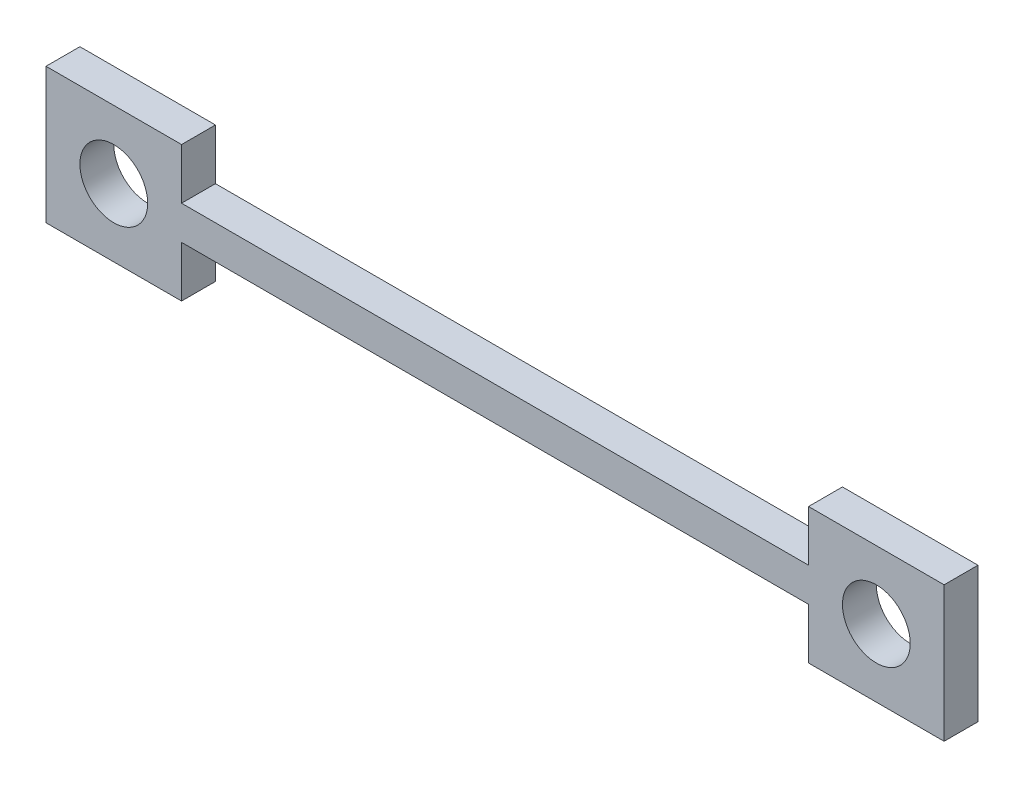
SolidWorks part; units mm, degrees
ref_plane "Front Plane" through (0, 0, 0) normal (0, 0, 1) x (1, 0, 0)
ref_plane "Top Plane" through (0, 0, 0) normal (0, 1, 0) x (1, 0, 0)
ref_plane "Right Plane" through (0, 0, 0) normal (1, 0, 0) x (0, 0, -1)
sketch "Sketch1" plane through (0, 0, 0) normal (0, 0, 1) x (1, 0, 0)
  line L0 (200, 50) -> (2050, 50)
  line L1 (-200, 200) -> (200, 200)
  line L2 (-200, 200) -> (-200, -200)
  line L3 (-200, -200) -> (200, -200)
  line L4 (200, 200) -> (200, 50)
  line L5 (200, -50) -> (2050, -50)
  line L6 (200, -50) -> (200, -200)
  line L7 (2050, -50) -> (2050, -200)
  line L9 (2050, 200) -> (2450, 200)
  line L10 (2050, 200) -> (2050, 50)
  line L11 (2050, -200) -> (2450, -200)
  line L12 (2450, 200) -> (2450, -200)
  circle A0 centre (0, 0) radius 100
  circle A1 centre (2250, 0) radius 100
  dimension "D2" = 200
  dimension "D3" = 200
  dimension "D4" = 0
  dimension "D1" = 2250
  dimension "D5" = 400
  dimension "D6" = 400
  dimension "D7" = 200
  dimension "D8" = 200
  dimension "D9" = 400
  dimension "D10" = 200
  dimension "D11" = 400
  dimension "D12" = 200
  dimension "D13" = 50
  dimension "D14" = 100
extrude "Boss-Extrude1" add sketch "Sketch1" along normal blind 100
